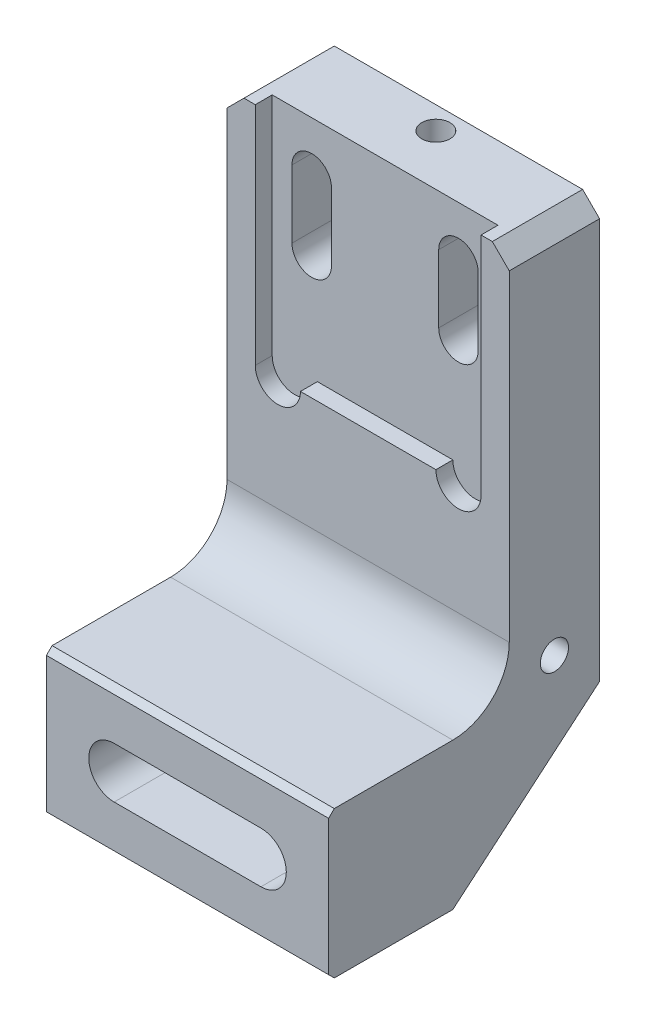
from build123d import *

# Parameters (mm, degrees)
SKETCH1_W             = 25
SKETCH1_H             = 48
BOSS_EXTRUDE1_DEPTH   = 4
SKETCH5_W             = 25
SKETCH5_H             = 24
BOSS_EXTRUDE3_DEPTH   = 13
SKETCH6_W             = 20
SKETCH6_H             = 40
CUT_EXTRUDE1_DEPTH    = 1.5
M3_TAPPED_HOLE1_D     = 2.5
M3_TAPPED_HOLE1_DEPTH = 11.5
M3_TAPPED_HOLE1_TIP   = 0.751075774
CHAMFER2_SIZE         = 1.5
CUT_EXTRUDE3_DEPTH    = 37.169738733
SKETCH18_R            = 2
CUT_EXTRUDE5_DEPTH    = 1.5
CUT_EXTRUDE6_DEPTH    = 37.169738733
CUT_EXTRUDE7_DEPTH    = 41.012498047
CUT_EXTRUDE8_DEPTH    = 15
FILLET2_R             = 5
CHAMFER4_SIZE         = 0.5


with BuildPart() as part:
    # Sketch1 → Boss-Extrude1 (new, symmetric)
    with BuildSketch(Plane.XY):
        Rectangle(SKETCH1_W, SKETCH1_H)
    extrude(amount=BOSS_EXTRUDE1_DEPTH, both=True)

    # Sketch5 → Boss-Extrude3 (add)
    with BuildSketch(Plane.XZ.offset(24)):
        with Locations((0, 8)):
            Rectangle(SKETCH5_W, SKETCH5_H)
    extrude(amount=-BOSS_EXTRUDE3_DEPTH)

    # Sketch6 → Cut-Extrude1 (cut)
    with BuildSketch(Plane.XY.offset(4)):
        with Locations((0, 24)):
            Rectangle(SKETCH6_W, SKETCH6_H)
    extrude(amount=-CUT_EXTRUDE1_DEPTH, mode=Mode.SUBTRACT)

    # M3 Tapped Hole1
    with Locations(Plane(origin=(0, 24, 0), x_dir=(1, 0, 0), z_dir=(0, 1, 0))):
        with Locations((0, 2)):
            Hole(M3_TAPPED_HOLE1_D / 2, depth=M3_TAPPED_HOLE1_DEPTH)
            with Locations((0, 0, -(M3_TAPPED_HOLE1_DEPTH + M3_TAPPED_HOLE1_TIP / 2))):  # 118° drill point
                Cone(0, M3_TAPPED_HOLE1_D / 2, M3_TAPPED_HOLE1_TIP, mode=Mode.SUBTRACT)

    # Chamfer2
    chamfer2_edges = [part.edges().sort_by_distance(p)[0] for p in [
        (-12.5, 24, 0),
        (12.5, 24, 0),
    ]]
    chamfer(chamfer2_edges, length=CHAMFER2_SIZE)

    # Sketch14 → Cut-Extrude3 (cut, through all)
    with BuildSketch(Plane(origin=(0, 0, -4), x_dir=(-1, 0, 0), z_dir=(0, 0, -1))):
        with BuildLine():
            Line((-4.75, 19.5), (-4.75, 13.5))
            ThreePointArc((-4.75, 13.5), (-6.5, 11.75), (-8.25, 13.5))
            Line((-8.25, 13.5), (-8.25, 19.5))
            ThreePointArc((-8.25, 19.5), (-6.5, 21.25), (-4.75, 19.5))
        make_face()
        with BuildLine():
            Line((8.25, 19.5), (8.25, 13.5))
            ThreePointArc((8.25, 13.5), (6.5, 11.75), (4.75, 13.5))
            Line((4.75, 13.5), (4.75, 19.5))
            ThreePointArc((4.75, 19.5), (6.5, 21.25), (8.25, 19.5))
        make_face()
    extrude(amount=-CUT_EXTRUDE3_DEPTH, mode=Mode.SUBTRACT)

    # Sketch15 → M3 Tapped Hole2 (revolve, cut)
    with BuildSketch(Plane(origin=(-12.5, -9, 0), x_dir=(0, 0, 1), z_dir=(0, 1, 0))):
        Polygon((0, 0), (0, 12.251075774), (1.25, 11.5), (1.25, 0), align=None)
    m3_tapped_hole2 = revolve(axis=Axis((-18.85, -9, 0), (1, 0, 0)), mode=Mode.SUBTRACT)

    # Sketch18 → Cut-Extrude5 (cut)
    with BuildSketch(Plane.XY.offset(4)):
        with Locations((-8, 4)):
            Circle(SKETCH18_R)
        with Locations((8, 4)):
            Circle(SKETCH18_R)
    extrude(amount=-CUT_EXTRUDE5_DEPTH, mode=Mode.SUBTRACT)

    # Sketch20 → Cut-Extrude6 (cut, through all)
    with BuildSketch(Plane(origin=(0, 0, -4), x_dir=(-1, 0, 0), z_dir=(0, 0, -1))):
        with BuildLine():
            Line((-6.5, -15.25), (6.5, -15.25))
            ThreePointArc((6.5, -15.25), (8.75, -17.5), (6.5, -19.75))
            Line((6.5, -19.75), (-6.5, -19.75))
            ThreePointArc((-6.5, -19.75), (-8.75, -17.5), (-6.5, -15.25))
        make_face()
    extrude(amount=-CUT_EXTRUDE6_DEPTH, mode=Mode.SUBTRACT)

    # Sketch21 → Cut-Extrude7 (cut, through all)
    with BuildSketch(Plane(origin=(12.5, 0, 0), x_dir=(0, 0, -1), z_dir=(1, 0, 0))):
        Polygon((-9, -24), (4, -13), (4, -24), align=None)
    extrude(amount=-CUT_EXTRUDE7_DEPTH, mode=Mode.SUBTRACT)

    # Sketch22 → Cut-Extrude8 (cut)
    with BuildSketch(Plane(origin=(0, 0, -4), x_dir=(-1, 0, 0), z_dir=(0, 0, -1))):
        with BuildLine():
            Line((-6.5, -13.5), (6.5, -13.5))
            ThreePointArc((6.5, -13.5), (10.5, -17.5), (6.5, -21.5))
            Line((6.5, -21.5), (-6.5, -21.5))
            ThreePointArc((-6.5, -21.5), (-10.5, -17.5), (-6.5, -13.5))
        make_face()
    extrude(amount=-CUT_EXTRUDE8_DEPTH, mode=Mode.SUBTRACT)

    # Fillet2
    fillet2_edges = [part.edges().sort_by_distance(p)[0] for p in [
        (0, -11, 4),
    ]]
    fillet(fillet2_edges, radius=FILLET2_R)

    # Mirror1: M3 Tapped Hole2 across plane
    add(m3_tapped_hole2.mirror(Plane(origin=(0, 0, 0), x_dir=(0, 0, 1), z_dir=(1, 0, 0))), mode=Mode.SUBTRACT)

    # Chamfer4
    chamfer4_edges = [part.edges().sort_by_distance(p)[0] for p in [
        (0, -24, 20),
        (0, -11, 20),
    ]]
    chamfer(chamfer4_edges, length=CHAMFER4_SIZE)


solid = part.part
